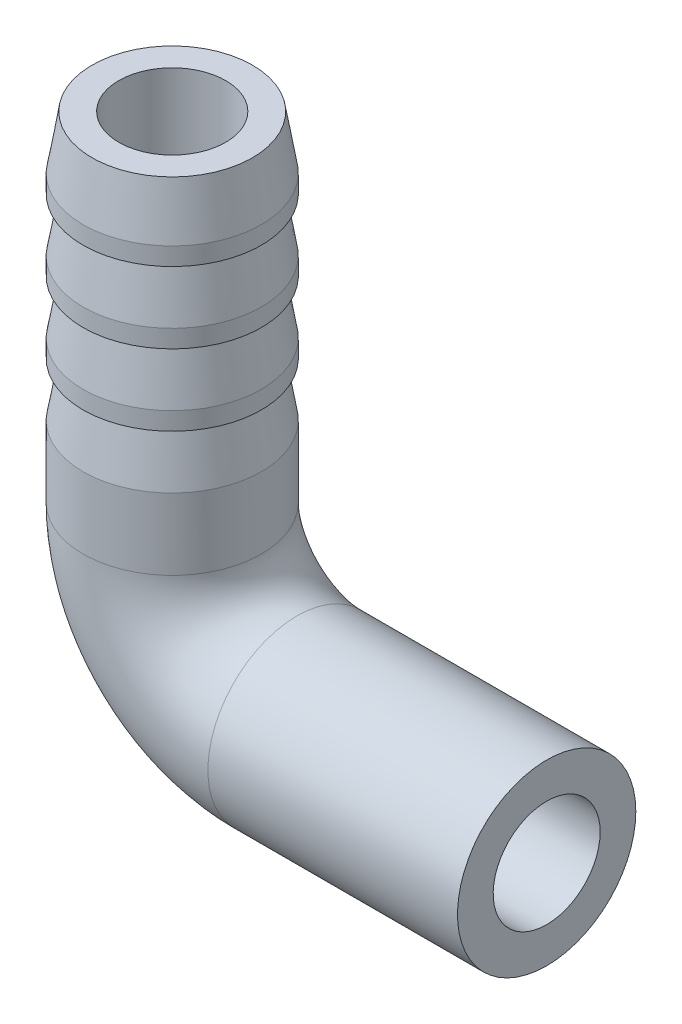
from build123d import *

# Parameters (mm, degrees)
CUT_EXTRUDE_1_REACH = 22.273
SKETCH_4_R          = 3
SKETCH_6_R          = 5
SKETCH_6_R_2        = 3


with BuildPart() as part:
    # 草图1 → 旋转1 (revolve)
    with BuildSketch(Plane.XY, mode=Mode.PRIVATE) as revolve_1_sk:
        Polygon((-5, 4), (-4.5, 7), (-5, 7), (-5, 8), (-4.5, 11), (-5, 11), (-5, 12), (-4.5, 15), (-5, 15), (-5, 16), (-4.5, 19), (0, 19), (0, 0), (-5, 0), align=None)
    revolve(revolve_1_sk.sketch.rotate(Axis((0, 0, 0), (0, 1, 0)), 270), axis=Axis((0, 0, 0), (0, 1, 0)))

    # 草图4 → 切除-拉伸1 (cut, up to next)
    with BuildSketch(Plane(origin=(0, 19, 0), x_dir=(1, 0, 0), z_dir=(0, 1, 0)), mode=Mode.PRIVATE) as cut_extrude_1_sk1:
        with Locations(Location((0, 0, 0), (0, 0, 180))):
            Circle(SKETCH_4_R)
    cut_extrude_1_tool1 = extrude(cut_extrude_1_sk1.sketch, amount=-CUT_EXTRUDE_1_REACH, mode=Mode.PRIVATE) & part.part
    add(cut_extrude_1_tool1.solids().sort_by_distance((0, 19, 0))[0], mode=Mode.SUBTRACT)

    # 扫描1: sweep along a path in 草图5
    with BuildLine(Plane.XY) as sweep_1_path:
        Line((21, -7), (7, -7))
        ThreePointArc((7, -7), (2.050252532, -4.949747468), (0, 0))
    # 草图6 → 扫描1 (sweep)
    with BuildSketch(Plane.XZ):
        Circle(SKETCH_6_R)
        Circle(SKETCH_6_R_2, mode=Mode.SUBTRACT)
    sweep(path=sweep_1_path.line)


solid = part.part
